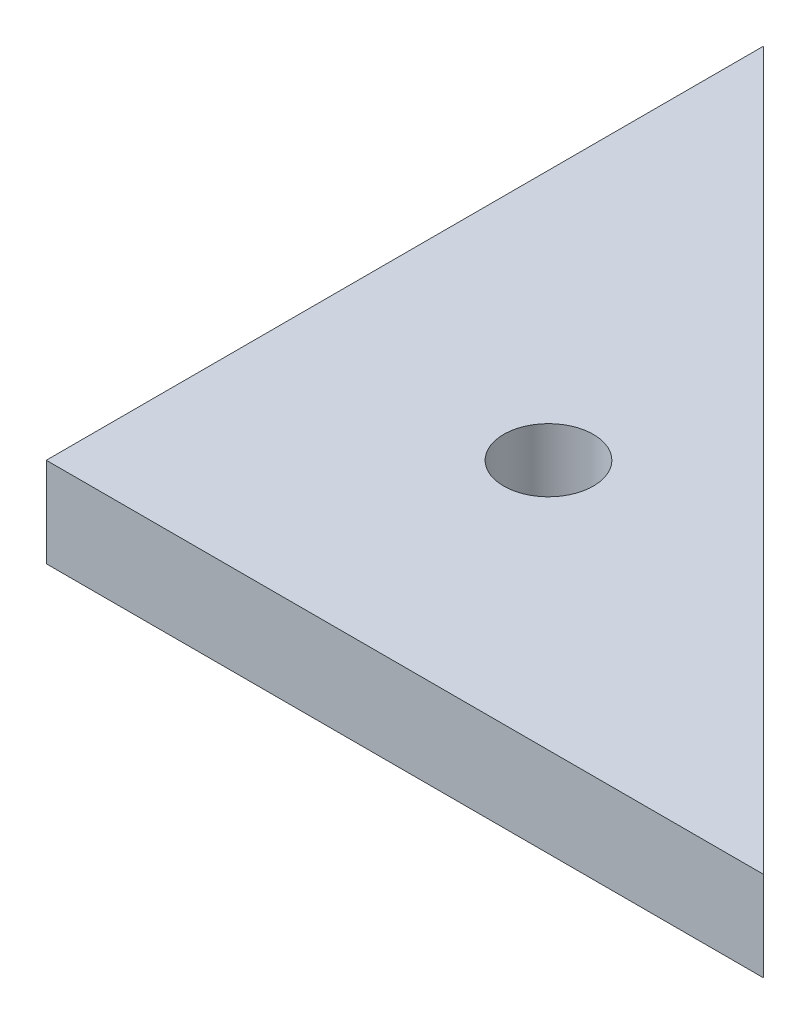
from build123d import *

# Parameters (mm, degrees)
EXTRUDE_1_DEPTH        = 5
HOLE_WIZARD_M6_1_D     = 5
HOLE_WIZARD_M6_1_DEPTH = 15
HOLE_WIZARD_M6_1_TIP   = 1.502151548


with BuildPart() as part:
    # 草图1 → 凸台-拉伸1 (new body)
    with BuildSketch(Plane(origin=(0, 0, 0), x_dir=(1, 0, 0), z_dir=(0, 1, 0))):
        Polygon((0, 40), (0, 0), (40, 0), align=None)
    extrude(amount=EXTRUDE_1_DEPTH)

    # M6 螺纹孔1
    with Locations(Plane(origin=(0, 5, 0), x_dir=(1, 0, 0), z_dir=(0, 1, 0))):
        with Locations((14, 14)):
            Hole(HOLE_WIZARD_M6_1_D / 2, depth=HOLE_WIZARD_M6_1_DEPTH)
            with Locations((0, 0, -(HOLE_WIZARD_M6_1_DEPTH + HOLE_WIZARD_M6_1_TIP / 2))):  # 118° drill point
                Cone(0, HOLE_WIZARD_M6_1_D / 2, HOLE_WIZARD_M6_1_TIP, mode=Mode.SUBTRACT)


solid = part.part
